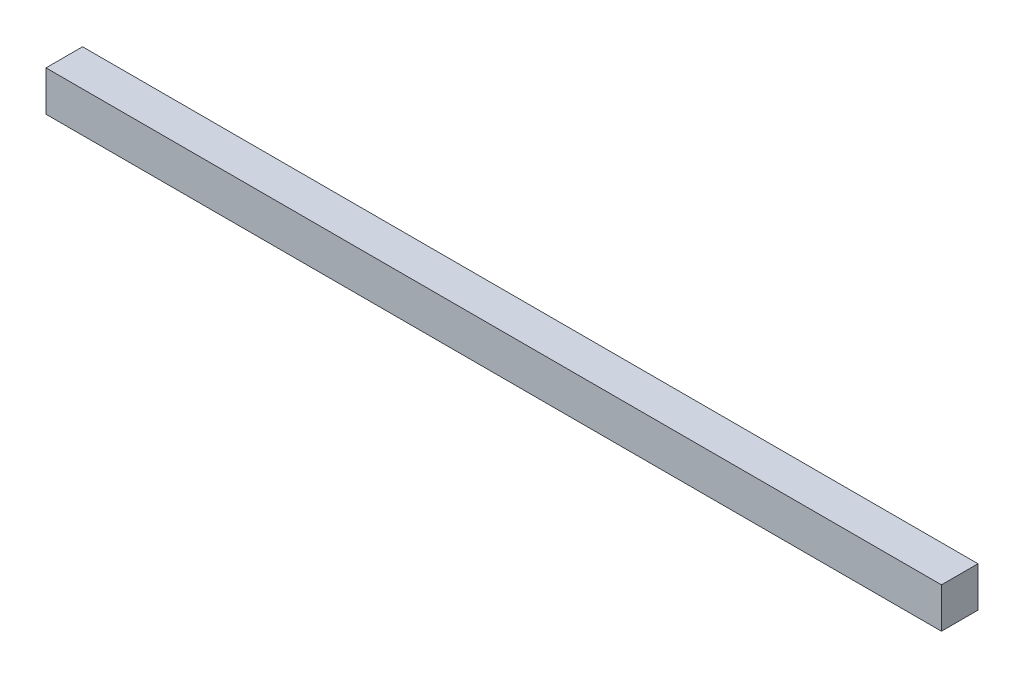
from build123d import *

# Parameters (mm, degrees)
SKETCH1_W           = 490
SKETCH1_H           = 22
BOSS_EXTRUDE1_DEPTH = 20


with BuildPart() as part:
    # Sketch1 → Boss-Extrude1 (new body)
    with BuildSketch(Plane.XY):
        with Locations((245, 11)):
            Rectangle(SKETCH1_W, SKETCH1_H)
    extrude(amount=BOSS_EXTRUDE1_DEPTH)


solid = part.part
